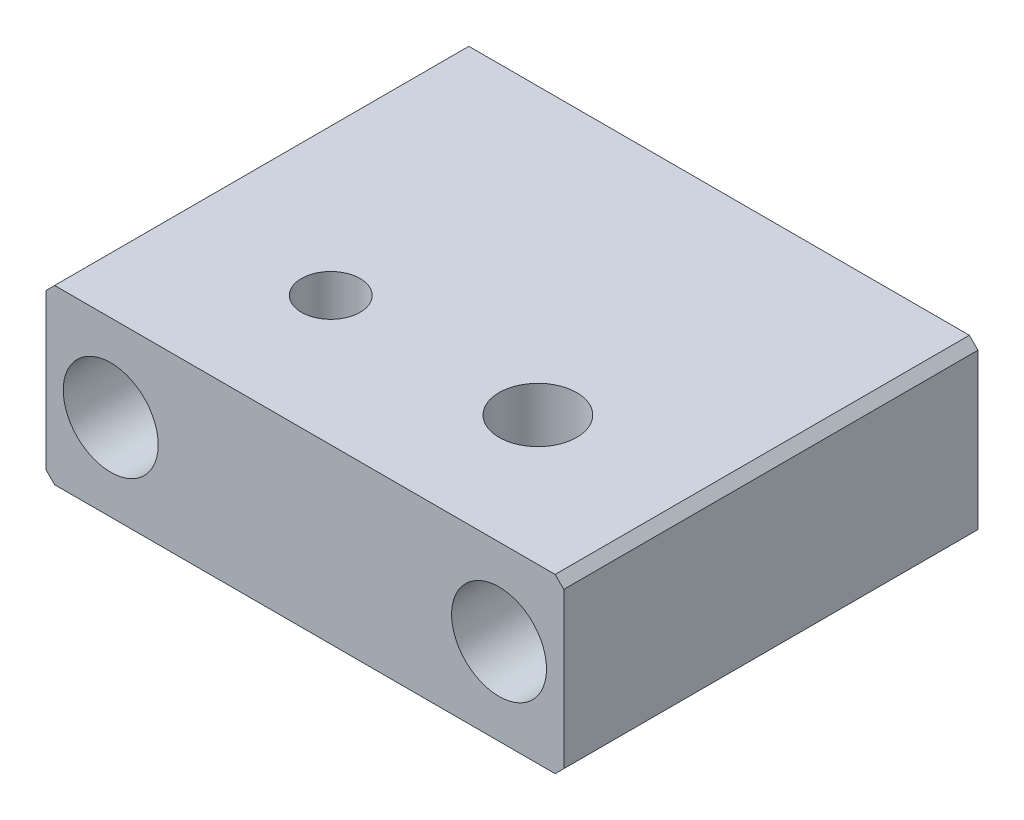
SolidWorks part; units mm, degrees
material "45"
ref_plane "Front Plane" through (0, 0, 0) normal (0, 0, 1) x (1, 0, 0)
ref_plane "Top Plane" through (0, 0, 0) normal (0, 1, 0) x (1, 0, 0)
ref_plane "Right Plane" through (0, 0, 0) normal (1, 0, 0) x (0, 0, -1)
sketch "Sketch1" plane through (0, 0, 0) normal (0, 0, 1) x (1, 0, 0)
  line L1 (-30, 10) -> (30, 10)
  line L2 (-30, 10) -> (-30, -10)
  line L3 (-30, -10) -> (30, -10)
  line L4 (30, 10) -> (30, -10)
  line L5 (-30, 10) -> (30, -10) construction
  line L6 (-30, -10) -> (30, 10) construction
  point P0 (0, 0)
  dimension "D1" = 20
  dimension "D2" = 60
extrude "Boss-Extrude1" add sketch "Sketch1" along normal blind 48
hole_wizard "CBORE for M6 Hex Socket Head Cap Screw1" positions "Sketch2" profile "Sketch3" counterbore size "M6" standard "ISO" end condition through all
sketch "Sketch2" plane through (0, 0, 48) normal (0, 0, 1) x (1, 0, 0)
  point P0 (-22.5, 0)
  point P2 (22.5, 0)
  dimension "D1" = 45
  dimension "D2" = 22.5
sketch "Sketch3" plane through (-22.5, 0, 48) normal (1, 0, 0) x (0, -1, 0)
  line L0 (0, 0) -> (0, 48)
  line L1 (0, 48) -> (3.3, 48)
  line L3 (3.3, 48) -> (3.3, 8)
  line L4 (3.3, 8) -> (5.5, 8)
  line L5 (5.5, 8) -> (5.5, 0)
  line L7 (5.5, 0) -> (0, 0)
  line L11 (0, -6.35) -> (0, 107.95) construction
  dimension "通孔孔直径" = 6.6
  dimension "通孔孔深度" = 48
  dimension "柱形沉头孔直径" = 11
  dimension "柱形沉头孔深度" = 8
hole_wizard "M8 Tapped Hole1" positions "Sketch4" profile "Sketch5" tap size "M8" standard "ISO" end condition through all
sketch "Sketch4" plane through (0, -10, 0) normal (0, -1, 0) x (1, 0, 0)
  line L0 (-30, 48) -> (30, 48) construction
  point P0 (-12, 33)
  dimension "D1" = 15
  dimension "D2" = 12
sketch "Sketch5" plane through (-12, -10, 33) normal (1, 0, 0) x (0, 0, -1)
  line L0 (0, 0) -> (0, 20)
  line L1 (0, 20) -> (3.4, 20)
  line L2 (3.4, 20) -> (3.4, 0)
  line L5 (3.4, 0) -> (0, 0)
  line L11 (0, -6.35) -> (0, 107.95) construction
  dimension "通孔螺纹孔钻头直径" = 6.8
  dimension "通孔螺纹孔钻头深度" = 20
cosmetic thread "Cosmetic Thread1" parameters "D2"=8
hole_wizard "M10x1.0 Tapped Hole1" positions "Sketch7" profile "Sketch8" tap size "M10x1.0" standard "ISO" end condition through all
sketch "Sketch7" plane through (0, -10, 0) normal (0, -1, 0) x (1, 0, 0)
  line L0 (-30, 48) -> (30, 48) construction
  circle A0 centre (-12, 33) radius 3.4 construction
  point P0 (12, 33)
  dimension "D1" = 24
  dimension "D2" = 15
sketch "Sketch8" plane through (12, -10, 33) normal (1, 0, 0) x (0, 0, -1)
  line L0 (0, 0) -> (0, 20)
  line L1 (0, 20) -> (4.5, 20)
  line L2 (4.5, 20) -> (4.5, 0)
  line L5 (4.5, 0) -> (0, 0)
  line L11 (0, -6.35) -> (0, 107.95) construction
  dimension "通孔螺纹孔钻头直径" = 9
  dimension "通孔螺纹孔钻头深度" = 20
cosmetic thread "Cosmetic Thread2" parameters "D2"=10
chamfer "Chamfer1" distance 1 angle 45 4 edges at (30, 10, 24) (30, -10, 24) (-30, 10, 24) (-30, -10, 24)
